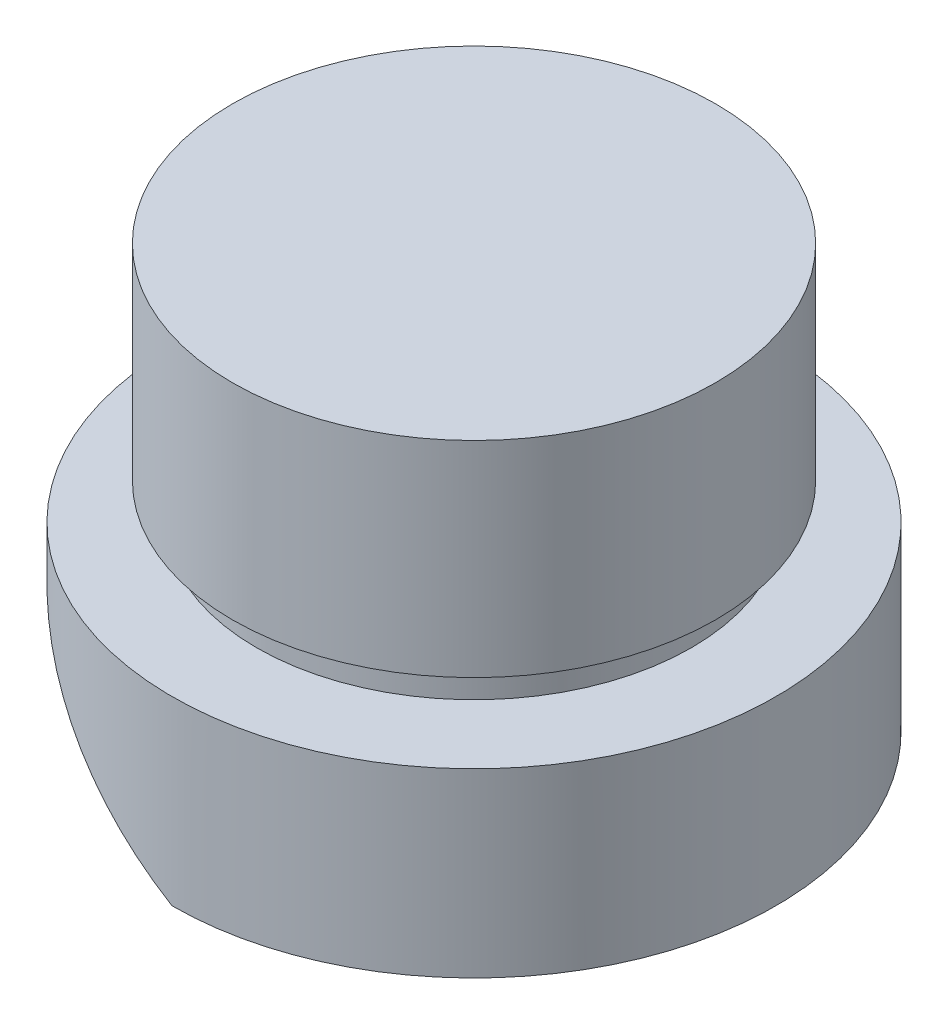
SolidWorks part; units mm, degrees
ref_plane "Front Plane" through (0, 0, 0) normal (0, 0, 1) x (1, 0, 0)
ref_plane "Top Plane" through (0, 0, 0) normal (0, 1, 0) x (1, 0, 0)
ref_plane "Right Plane" through (0, 0, 0) normal (1, 0, 0) x (0, 0, -1)
sketch "Sketch1" plane through (0, 0, 0) normal (0, 0, 1) x (1, 0, 0)
  line L0 (0, 13.7119) -> (0, -13.6011) construction
  line L2 (0, 17.8255) -> (-20, 17.8255)
  line L3 (0, 17.8255) -> (0, 0.8255)
  line L4 (0, 0.8255) -> (-20, 0.8255)
  line L5 (-20, 17.8255) -> (-20, 0.8255)
  line L6 (0, 0.8255) -> (-18, 0.8255)
  line L7 (0, 0.8255) -> (0, -2.1745)
  line L8 (0, -2.1745) -> (-18, -2.1745)
  line L9 (-18, 0.8255) -> (-18, -2.1745)
  line L10 (0, -2.1745) -> (-25, -2.1745)
  line L11 (0, -2.1745) -> (0, -17.1745)
  line L12 (0, -17.1745) -> (-25, -17.1745)
  line L13 (-25, -2.1745) -> (-25, -17.1745)
  dimension "D1" = 20
  dimension "D2" = 17
  dimension "D3" = 3
  dimension "D4" = 18
  dimension "D5" = 25
  dimension "D6" = 35
revolve "Revolve2" add sketch "Sketch1" angle 360 about L0
sketch "Sketch3" plane through (0, 0, 0) normal (0, 0, 1) x (1, 0, 0)
  line L0 (0, 24.1019) -> (0, -23.9392)
  line L1 (0, -17.1745) -> (-25, -17.1745)
  line L2 (-25, -17.1745) -> (25, -17.1745) construction
  line L4 (-25, -2.1745) -> (0, -17.1745)
  line L5 (-25, -2.1745) -> (-25, -17.1745)
extrude "Cut-Extrude1" cut sketch "Sketch3" against normal through all both and the other way through all contours L4 L5 L1
